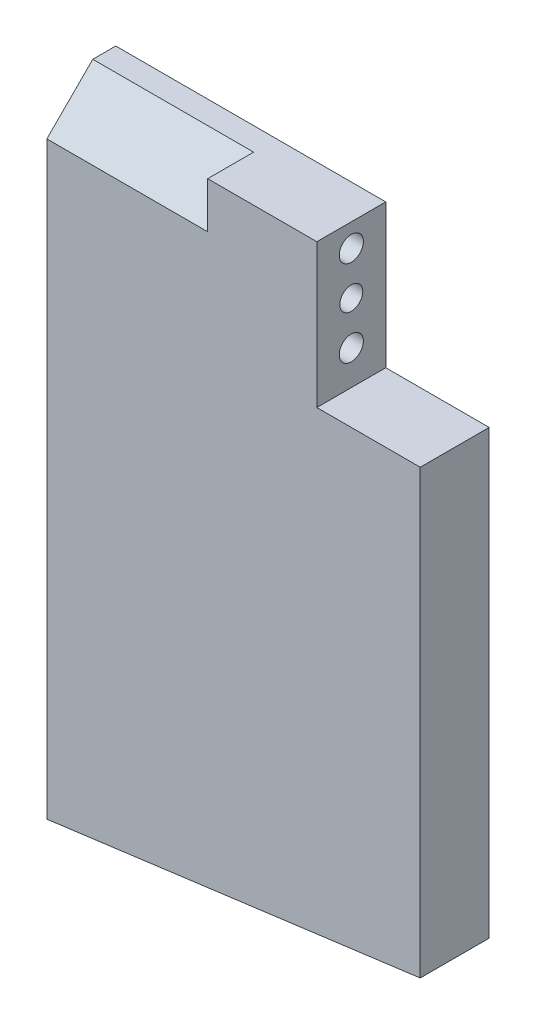
SolidWorks part; units mm, degrees
ref_plane "Front Plane" through (0, 0, 0) normal (0, 0, 1) x (1, 0, 0)
ref_plane "Top Plane" through (0, 0, 0) normal (0, 1, 0) x (1, 0, 0)
ref_plane "Right Plane" through (0, 0, 0) normal (1, 0, 0) x (0, 0, -1)
sketch "Sketch1" plane through (0, 0, 0) normal (0, 1, 0) x (1, 0, 0)
  line L1 (-32.5, 6) -> (32.5, 6)
  line L2 (-32.5, 6) -> (-32.5, -6)
  line L3 (-32.5, -6) -> (32.5, -6)
  line L4 (32.5, 6) -> (32.5, -6)
  line L5 (-32.5, 6) -> (32.5, -6) construction
  line L6 (-32.5, -6) -> (32.5, 6) construction
  point P0 (0, 0)
  dimension "D1" = 65
  dimension "D2" = 12
extrude "Boss-Extrude1" add sketch "Sketch1" along normal mid plane 102
sketch "Sketch4" plane through (0, 0, 6) normal (0, 0, 1) x (1, 0, 0)
  line L0 (-32.5, -51) -> (32.5, -51) construction
  line L1 (-32.5, -51) -> (32.5, -51)
  line L2 (32.5, -51) -> (-32.5, -59.5574)
  line L3 (-32.5, -51) -> (-32.5, -59.5574)
  dimension "D1" = 7.5
extrude "Boss-Extrude2" add sketch "Sketch4" against normal up to surface (12 mm away) up to face at (0, 0, -6)
sketch "Sketch3" plane through (0, 0, 6) normal (0, 0, 1) x (1, 0, 0)
  line L1 (32.5, 51) -> (14.5, 51)
  line L2 (32.5, 51) -> (32.5, 26)
  line L3 (32.5, 26) -> (14.5, 26)
  line L4 (14.5, 51) -> (14.5, 26)
  dimension "D1" = 25
  dimension "D2" = 18
extrude "Cut-Extrude2" cut sketch "Sketch3" against normal through all
hole_wizard "M5 Tapped Hole1" positions "Sketch6" profile "Sketch5" tap size "M5" standard "Gb"
sketch "Sketch6" plane through (7.1536, -54.3369, 0) normal (0.1305, -0.9914, 0) x (-0.9914, -0.1305, 0)
  line L0 (-25.5651, -6) -> (-25.5651, 6) construction
  point P0 (-18.0651, 0)
  point P2 (6.9349, 0)
  point P4 (31.9349, 0)
  dimension "D1" = 25
  dimension "D2" = 25
  dimension "D3" = 7.5
sketch "Sketch5" plane through (25.0642, -51.9789, 0) normal (0, 0, 1) x (0.9914, 0.1305, 0)
  line L0 (0, 0) -> (0, 13.6618)
  line L1 (0, 13.6618) -> (2.1, 12.4)
  line L2 (2.1, 12.4) -> (2.1, 0)
  line L5 (2.1, 0) -> (0, 0)
  line L10 (0, 13.6618) -> (-2.1, 12.4) construction
  line L11 (0, -6.35) -> (0, 107.95) construction
  dimension "螺纹孔钻头直径" = 4.2
  dimension "螺纹孔钻头深度" = 12.4
  dimension "导头角度" = 118
cosmetic thread "Hole Thread2" parameters "D1"=10, "D2"=5
cosmetic thread "Hole Thread3" parameters "D1"=10, "D2"=5
cosmetic thread "Hole Thread4" parameters "D1"=10, "D2"=5
hole_wizard "M5 Tapped Hole2" positions "Sketch8" profile "Sketch7" tap size "M5" standard "Gb"
sketch "Sketch8" plane through (-32.5, 0, 0) normal (-1, 0, 0) x (0, 0, 1)
  line L0 (-6, 51) -> (6, 51) construction
  point P0 (0, 43)
  point P2 (0, 3)
  point P4 (0, -37)
  dimension "D1" = 8
  dimension "D2" = 40
  dimension "D3" = 40
sketch "Sketch7" plane through (-32.5, 43, 0) normal (0, 1, 0) x (0, 0, 1)
  line L0 (0, 0) -> (0, 13.6618)
  line L1 (0, 13.6618) -> (2.1, 12.4)
  line L2 (2.1, 12.4) -> (2.1, 0)
  line L5 (2.1, 0) -> (0, 0)
  line L10 (0, 13.6618) -> (-2.1, 12.4) construction
  line L11 (0, -6.35) -> (0, 107.95) construction
  dimension "螺纹孔钻头直径" = 4.2
  dimension "螺纹孔钻头深度" = 12.4
  dimension "导头角度" = 118
cosmetic thread "Hole Thread5" parameters "D1"=10, "D2"=5
cosmetic thread "Hole Thread6" parameters "D1"=10, "D2"=5
cosmetic thread "Hole Thread7" parameters "D1"=10, "D2"=5
hole_wizard "M5 Tapped Hole3" positions "Sketch10" profile "Sketch9" tap size "M5" standard "Gb"
sketch "Sketch10" plane through (14.5, 0, 0) normal (1, 0, 0) x (0, 0, -1)
  line L0 (6, 51) -> (-6, 51) construction
  point P0 (0, 47)
  point P2 (0, 32)
  dimension "D1" = 4
  dimension "D2" = 15
sketch "Sketch9" plane through (14.5, 47, 0) normal (0, 1, 0) x (0, 0, -1)
  line L0 (0, 0) -> (0, 13.6618)
  line L1 (0, 13.6618) -> (2.1, 12.4)
  line L2 (2.1, 12.4) -> (2.1, 0)
  line L5 (2.1, 0) -> (0, 0)
  line L10 (0, 13.6618) -> (-2.1, 12.4) construction
  line L11 (0, -6.35) -> (0, 107.95) construction
  dimension "螺纹孔钻头直径" = 4.2
  dimension "螺纹孔钻头深度" = 12.4
  dimension "导头角度" = 118
cosmetic thread "Hole Thread8" parameters "D1"=10, "D2"=5
cosmetic thread "Hole Thread9" parameters "D1"=10, "D2"=5
sketch "Sketch12" plane through (-32.5, 0, 0) normal (-1, 0, 0) x (0, 0, 1)
  line L0 (-2, 51) -> (6, 51)
  line L1 (6, 51) -> (6, 43)
  line L2 (6, 43) -> (-2, 51)
  line L5 (-6, 51) -> (6, 51) construction
  line L6 (6, 51) -> (6, -59.5574) construction
  dimension "D1" = 45
  dimension "D2" = 8
extrude "Cut-Extrude3" cut sketch "Sketch12" against normal blind 28
hole_wizard "Ø4.0 (4) Diameter Hole1" positions "Sketch14" profile "Sketch13" hole size "Ø4.0" standard "Gb"
sketch "Sketch14" plane through (14.5, 0, 0) normal (1, 0, 0) x (0, 0, -1)
  circle A0 centre (0, 32) radius 2.1 construction
  point P0 (0, 39.5)
  dimension "D1" = 7.5
sketch "Sketch13" plane through (14.5, 39.5, 0) normal (0, 1, 0) x (0, 0, -1)
  line L0 (0, 0) -> (0, 9.2017)
  line L1 (0, 9.2017) -> (2, 8)
  line L2 (2, 8) -> (2, 0)
  line L5 (2, 0) -> (0, 0)
  line L10 (0, 9.2017) -> (-2, 8) construction
  line L11 (0, -6.35) -> (0, 107.95) construction
  dimension "孔直径" = 4
  dimension "孔深度" = 8
  dimension "导头角度" = 118
